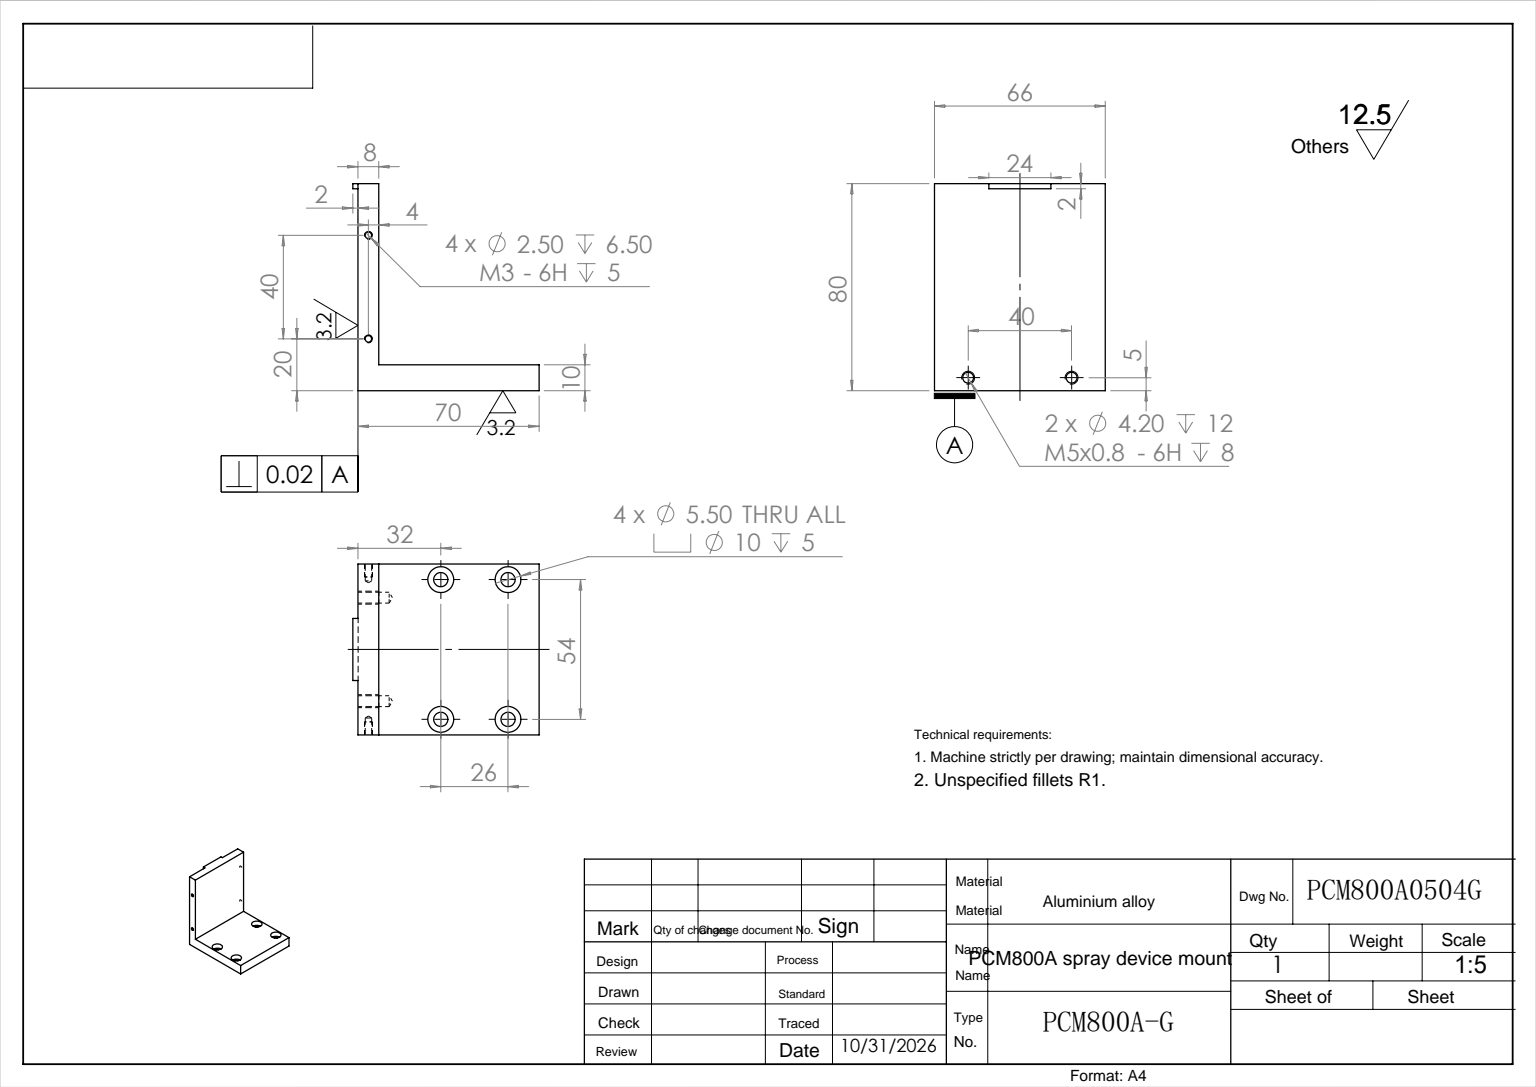
from build123d import *

# Parameters (mm, degrees)
SKETCH_1_W                   = 50
SKETCH_1_H                   = 66
EXTRUDE_1_DEPTH              = 10
HOLE_WIZARD_M5_1_D           = 5.5
HOLE_WIZARD_M5_1_CBORE_D     = 10
HOLE_WIZARD_M5_1_CBORE_DEPTH = 5
SKETCH_4_W                   = 10
SKETCH_4_H                   = 66
EXTRUDE_2_DEPTH              = 20
M5X0_8_2_D                   = 4.2
M5X0_8_2_DEPTH               = 12
M5X0_8_2_TIP                 = 1.2618073
SKETCH_12_W                  = 8
SKETCH_12_H                  = 66
EXTRUDE_3_DEPTH              = 70
SKETCH_14_W                  = 2
SKETCH_14_H                  = 24
EXTRUDE_4_DEPTH              = 2
HOLE_WIZARD_M3_1_AT_2_COUNT  = 2
HOLE_WIZARD_M3_1_AT_2_PITCH  = 40


with BuildPart() as part:
    # 草图1 → 拉伸1 (new body)
    with BuildSketch(Plane.XY):
        with Locations((25, 33)):
            Rectangle(SKETCH_1_W, SKETCH_1_H)
    extrude(amount=EXTRUDE_1_DEPTH)

    # M5 凹头盖螺钉的柱形沉头孔1 (through all)
    with Locations(Plane(origin=(0, 0, 0), x_dir=(-1, 0, 0), z_dir=(0, 0, -1))):
        with Locations((-38, 6), (-38, 60), (-12, 60), (-12, 6)):
            CounterBoreHole(HOLE_WIZARD_M5_1_D / 2, HOLE_WIZARD_M5_1_CBORE_D / 2, HOLE_WIZARD_M5_1_CBORE_DEPTH)

    # 草图4 → 拉伸2 (add)
    with BuildSketch(Plane(origin=(50, 0, 0), x_dir=(0, 0, -1), z_dir=(1, 0, 0))):
        with Locations((-5, 33)):
            Rectangle(SKETCH_4_W, SKETCH_4_H)
    extrude(amount=EXTRUDE_2_DEPTH)

    # M5x0.8 螺纹孔2
    with Locations(Plane(origin=(70, 0, 0), x_dir=(0, 0, -1), z_dir=(1, 0, 0))):
        with Locations((-5, 53), (-5, 13)):
            Hole(M5X0_8_2_D / 2, depth=M5X0_8_2_DEPTH)
            with Locations((0, 0, -(M5X0_8_2_DEPTH + M5X0_8_2_TIP / 2))):  # 118° drill point
                Cone(0, M5X0_8_2_D / 2, M5X0_8_2_TIP, mode=Mode.SUBTRACT)

    # 草图12 → 拉伸3 (add)
    with BuildSketch(Plane(origin=(0, 0, 0), x_dir=(-1, 0, 0), z_dir=(0, 0, -1))):
        with Locations((-66, 33)):
            Rectangle(SKETCH_12_W, SKETCH_12_H)
    extrude(amount=EXTRUDE_3_DEPTH)

    # 草图14 → 拉伸4 (add)
    with BuildSketch(Plane(origin=(70, 0, 0), x_dir=(0, 0, -1), z_dir=(1, 0, 0))):
        with Locations((69, 33)):
            Rectangle(SKETCH_14_W, SKETCH_14_H)
    extrude(amount=EXTRUDE_4_DEPTH)

    # 草图15 → M3 螺纹孔1 (revolve, cut)
    with BuildSketch(Plane(origin=(66, 0, -10), x_dir=(0, 0, -1), z_dir=(1, 0, 0))):
        Polygon((0, 0), (0, 7.251075774), (1.25, 6.5), (1.25, 0), align=None)
    hole_wizard_m3_1 = revolve(axis=Axis((66, -6.35, -10), (0, 1, 0)), mode=Mode.SUBTRACT)

    # M3 螺纹孔1 at 2: M3 螺纹孔1 ×2
    with Locations(*[(0, 0, -i * HOLE_WIZARD_M3_1_AT_2_PITCH) for i in range(1, HOLE_WIZARD_M3_1_AT_2_COUNT)]):
        add(hole_wizard_m3_1, mode=Mode.SUBTRACT)

    # 镜向1: M3 螺纹孔1 across plane
    add(hole_wizard_m3_1.mirror(Plane(origin=(0, 33, 0), x_dir=(0, 0, 1), z_dir=(0, -1, 0))), mode=Mode.SUBTRACT)

    # 镜向1 copy 1 sketch → 镜向1 copy 1 (revolve, cut)
    with BuildSketch(Plane(origin=(66, 66, -50), x_dir=(0, 0, -1), z_dir=(1, 0, 0))):
        Polygon((0, 0), (0, -7.251075774), (1.25, -6.5), (1.25, 0), align=None)
    revolve(axis=Axis((66, 72.35, -50), (0, 1, 0)), mode=Mode.SUBTRACT)


solid = part.part
